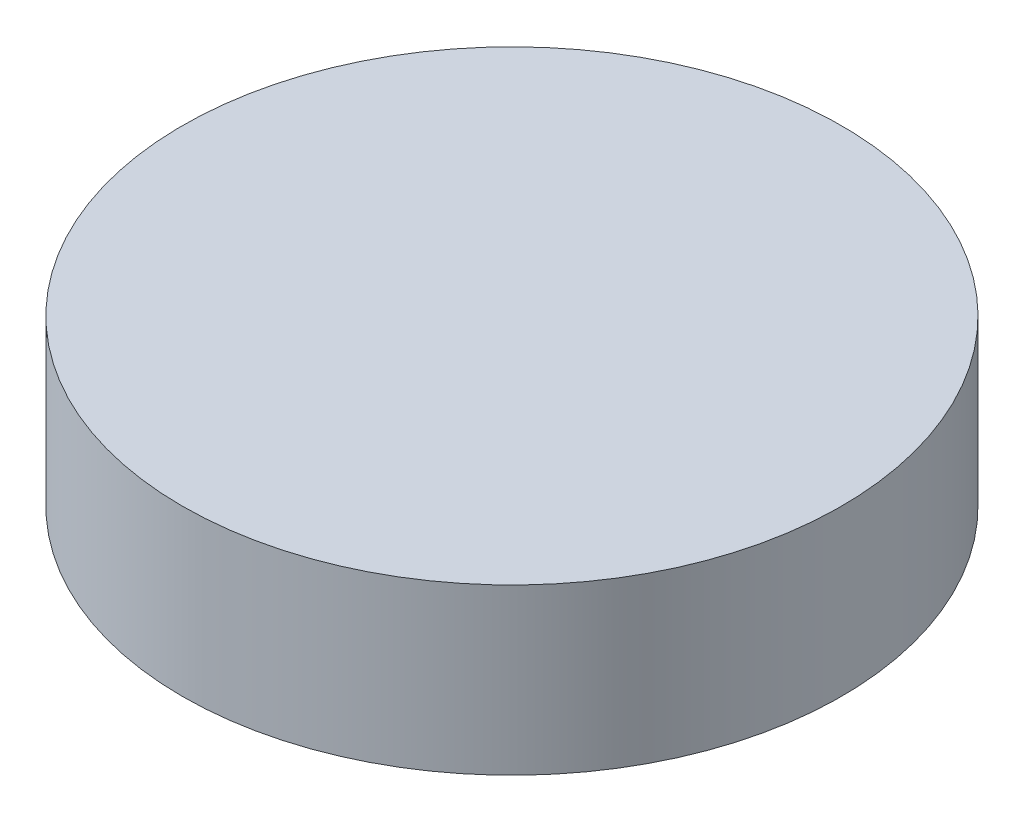
from build123d import *

# Parameters (mm, degrees)
SKETCH1_R           = 4
BOSS_EXTRUDE1_DEPTH = 2


with BuildPart() as part:
    # Sketch1 → Boss-Extrude1 (new body)
    with BuildSketch(Plane(origin=(0, 0, 0), x_dir=(1, 0, 0), z_dir=(0, 1, 0))):
        with Locations(Location((0, 0, 0), (0, 0, 270))):
            Circle(SKETCH1_R)
    extrude(amount=BOSS_EXTRUDE1_DEPTH)


solid = part.part
